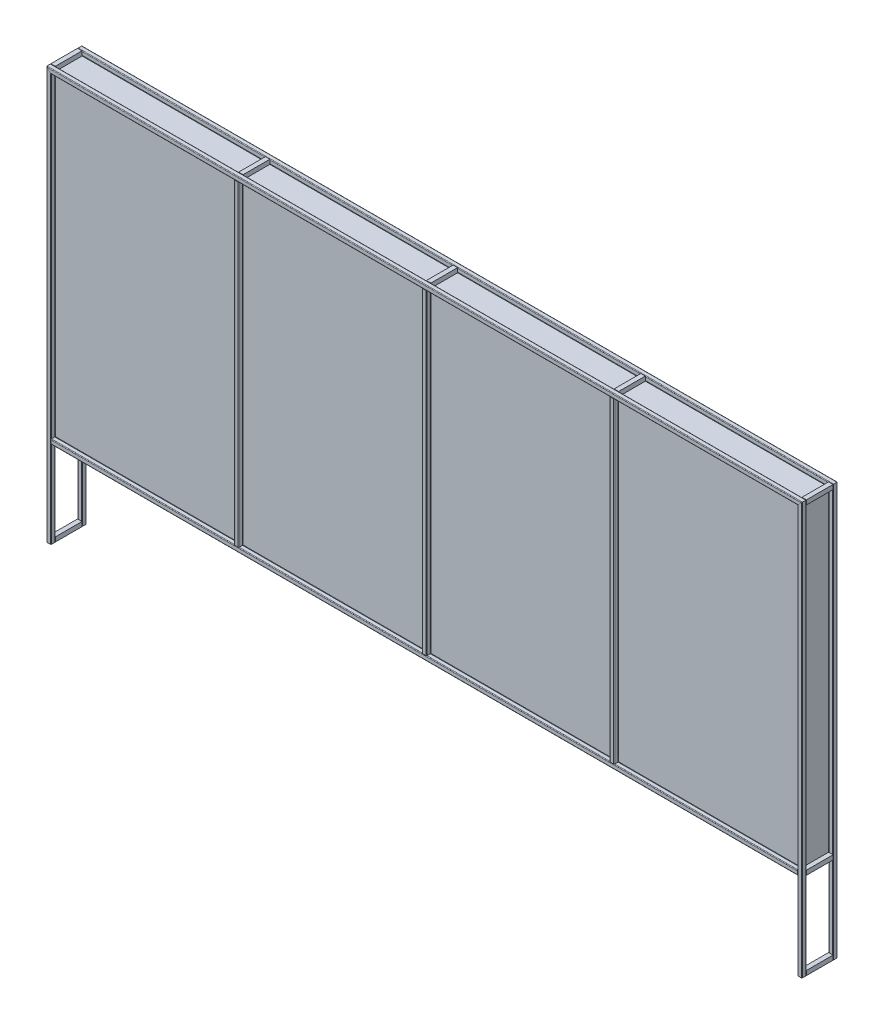
from build123d import *

# Parameters (mm, degrees)
GB_6728_1986_025_X_25_X_1_75_1_DEPTH        = 2318.67766953
GB_6728_1986_025_X_25_X_1_75_1_2_DEPTH      = 4252.355339059
GB_6728_1986_025_X_25_X_1_75_1_3_DEPTH      = 2300
GB_6728_1986_025_X_25_X_1_75_1_3_DEPTH_BACK = 18.67766953
GB_6728_1986_025_X_25_X_1_75_1_4_DEPTH      = 4217
GB_6728_1986_025_X_25_X_1_75_1_5_DEPTH      = 1802
GB_6728_1986_025_X_25_X_1_75_1_6_DEPTH      = 1802
GB_6728_1986_025_X_25_X_1_75_1_7_DEPTH      = 1802
PATTERN_LINEAR_1_COUNT                      = 2
PATTERN_LINEAR_1_PITCH                      = 175
SKETCH_2_W                                  = 25
SKETCH_2_H                                  = 25
EXTRUDE_1_DEPTH                             = 150
EXTRUDE_1_2_DEPTH                           = 150
EXTRUDE_1_3_DEPTH                           = 150
EXTRUDE_1_4_DEPTH                           = 150
EXTRUDE_1_5_DEPTH                           = 150
EXTRUDE_1_6_DEPTH                           = 150
EXTRUDE_1_7_DEPTH                           = 150
EXTRUDE_1_8_DEPTH                           = 150
EXTRUDE_1_9_DEPTH                           = 150
EXTRUDE_1_10_DEPTH                          = 150
EXTRUDE_1_11_DEPTH                          = 150
EXTRUDE_1_12_DEPTH                          = 150
SKETCH_3_W                                  = 1028.75
SKETCH_3_H                                  = 1775
EXTRUDE_2_DEPTH                             = 150
PATTERN_LINEAR_3_COUNT                      = 4
PATTERN_LINEAR_3_PITCH                      = 1053.75


with BuildPart() as part:
    # Sketch1 on segment 1 (carried to segment 1) → Gb／6728-1986方形空心型钢 025 X 25 X 1.75(1) (new body)
    with BuildSketch(Plane(origin=(2107.5, 0, 0), x_dir=(-1, 0, 0), z_dir=(0, 1, 0))):
        with BuildLine():
            Line((-9, -12.5), (9, -12.5))
            ThreePointArc((9, -12.5), (11.474873734, -11.474873734), (12.5, -9))
            Line((12.5, -9), (12.5, 9))
            ThreePointArc((12.5, 9), (11.474873734, 11.474873734), (9, 12.5))
            Line((9, 12.5), (-9, 12.5))
            ThreePointArc((-9, 12.5), (-11.474873734, 11.474873734), (-12.5, 9))
            Line((-12.5, 9), (-12.5, -9))
            ThreePointArc((-12.5, -9), (-11.474873734, -11.474873734), (-9, -12.5))
        make_face()
        with BuildLine():
            Line((-9, -10.75), (9, -10.75))
            ThreePointArc((9, -10.75), (10.237436867, -10.237436867), (10.75, -9))
            Line((10.75, -9), (10.75, 9))
            ThreePointArc((10.75, 9), (10.237436867, 10.237436867), (9, 10.75))
            Line((9, 10.75), (-9, 10.75))
            ThreePointArc((-9, 10.75), (-10.237436867, 10.237436867), (-10.75, 9))
            Line((-10.75, 9), (-10.75, -9))
            ThreePointArc((-10.75, -9), (-10.237436867, -10.237436867), (-9, -10.75))
        make_face(mode=Mode.SUBTRACT)
    extrude(amount=GB_6728_1986_025_X_25_X_1_75_1_DEPTH)

    # Gb／6728-1986方形空心型钢 025 X 25 X 1.75(1) mitre 1
    split(bisect_by=Plane(origin=(2107.5, 2300, 0), x_dir=(0.707106781, 0.707106781, 0), z_dir=(0.707106781, -0.707106781, 0)), keep=Keep.TOP)


with BuildPart() as body_2:
    # Sketch1 on segment 2 (carried to segment 2) → Gb_6728-1986_ 025 X 25 X 1.75_1 2 (new body)
    with BuildSketch(Plane(origin=(2126.17766953, 2300, 0), x_dir=(0, -1, 0), z_dir=(-1, 0, 0))):
        with BuildLine():
            Line((-9, -12.5), (9, -12.5))
            ThreePointArc((9, -12.5), (11.474873734, -11.474873734), (12.5, -9))
            Line((12.5, -9), (12.5, 9))
            ThreePointArc((12.5, 9), (11.474873734, 11.474873734), (9, 12.5))
            Line((9, 12.5), (-9, 12.5))
            ThreePointArc((-9, 12.5), (-11.474873734, 11.474873734), (-12.5, 9))
            Line((-12.5, 9), (-12.5, -9))
            ThreePointArc((-12.5, -9), (-11.474873734, -11.474873734), (-9, -12.5))
        make_face()
        with BuildLine():
            Line((-9, -10.75), (9, -10.75))
            ThreePointArc((9, -10.75), (10.237436867, -10.237436867), (10.75, -9))
            Line((10.75, -9), (10.75, 9))
            ThreePointArc((10.75, 9), (10.237436867, 10.237436867), (9, 10.75))
            Line((9, 10.75), (-9, 10.75))
            ThreePointArc((-9, 10.75), (-10.237436867, 10.237436867), (-10.75, 9))
            Line((-10.75, 9), (-10.75, -9))
            ThreePointArc((-10.75, -9), (-10.237436867, -10.237436867), (-9, -10.75))
        make_face(mode=Mode.SUBTRACT)
    extrude(amount=GB_6728_1986_025_X_25_X_1_75_1_2_DEPTH)

    # Gb_6728-1986_ 025 X 25 X 1.75_1 2 mitre
    split(bisect_by=Plane(origin=(-2107.5, 2300, 0), x_dir=(-0.707106781, 0.707106781, 0), z_dir=(0.707106781, 0.707106781, 0)), keep=Keep.TOP)

    # Gb_6728-1986_ 025 X 25 X 1.75_1 2 mi 2
    split(bisect_by=Plane(origin=(2107.5, 2300, 0), x_dir=(-0.707106781, -0.707106781, 0), z_dir=(-0.707106781, 0.707106781, 0)), keep=Keep.TOP)


with BuildPart() as body_3:
    # Sketch1 → Gb_6728-1986_ 025 X 25 X 1.75_1 3 (new, two sides: drawn at the far end of the back side and taken through both)
    with BuildSketch(Plane(origin=(-2107.5, 2300, 0), x_dir=(1, 0, 0), z_dir=(0, -1, 0)).offset(-GB_6728_1986_025_X_25_X_1_75_1_3_DEPTH_BACK)):
        with BuildLine():
            Line((-9, -12.5), (9, -12.5))
            ThreePointArc((9, -12.5), (11.474873734, -11.474873734), (12.5, -9))
            Line((12.5, -9), (12.5, 9))
            ThreePointArc((12.5, 9), (11.474873734, 11.474873734), (9, 12.5))
            Line((9, 12.5), (-9, 12.5))
            ThreePointArc((-9, 12.5), (-11.474873734, 11.474873734), (-12.5, 9))
            Line((-12.5, 9), (-12.5, -9))
            ThreePointArc((-12.5, -9), (-11.474873734, -11.474873734), (-9, -12.5))
        make_face()
        with BuildLine():
            Line((-9, -10.75), (9, -10.75))
            ThreePointArc((9, -10.75), (10.237436867, -10.237436867), (10.75, -9))
            Line((10.75, -9), (10.75, 9))
            ThreePointArc((10.75, 9), (10.237436867, 10.237436867), (9, 10.75))
            Line((9, 10.75), (-9, 10.75))
            ThreePointArc((-9, 10.75), (-10.237436867, 10.237436867), (-10.75, 9))
            Line((-10.75, 9), (-10.75, -9))
            ThreePointArc((-10.75, -9), (-10.237436867, -10.237436867), (-9, -10.75))
        make_face(mode=Mode.SUBTRACT)
    extrude(amount=GB_6728_1986_025_X_25_X_1_75_1_3_DEPTH + GB_6728_1986_025_X_25_X_1_75_1_3_DEPTH_BACK)

    # Gb_6728-1986_ 025 X 25 X 1.75_1 3 mitre
    split(bisect_by=Plane(origin=(-2107.5, 2300, 0), x_dir=(0.707106781, -0.707106781, 0), z_dir=(-0.707106781, -0.707106781, 0)), keep=Keep.TOP)


with BuildPart() as body_4:
    # Sketch1 on segment 4 (carried to segment 4) → Gb_6728-1986_ 025 X 25 X 1.75_1 4 (new body)
    with BuildSketch(Plane(origin=(-2108.5, 500, 0), x_dir=(0, 1, 0), z_dir=(1, 0, 0))):
        with BuildLine():
            Line((-9, -12.5), (9, -12.5))
            ThreePointArc((9, -12.5), (11.474873734, -11.474873734), (12.5, -9))
            Line((12.5, -9), (12.5, 9))
            ThreePointArc((12.5, 9), (11.474873734, 11.474873734), (9, 12.5))
            Line((9, 12.5), (-9, 12.5))
            ThreePointArc((-9, 12.5), (-11.474873734, 11.474873734), (-12.5, 9))
            Line((-12.5, 9), (-12.5, -9))
            ThreePointArc((-12.5, -9), (-11.474873734, -11.474873734), (-9, -12.5))
        make_face()
        with BuildLine():
            Line((-9, -10.75), (9, -10.75))
            ThreePointArc((9, -10.75), (10.237436867, -10.237436867), (10.75, -9))
            Line((10.75, -9), (10.75, 9))
            ThreePointArc((10.75, 9), (10.237436867, 10.237436867), (9, 10.75))
            Line((9, 10.75), (-9, 10.75))
            ThreePointArc((-9, 10.75), (-10.237436867, 10.237436867), (-10.75, 9))
            Line((-10.75, 9), (-10.75, -9))
            ThreePointArc((-10.75, -9), (-10.237436867, -10.237436867), (-9, -10.75))
        make_face(mode=Mode.SUBTRACT)
    extrude(amount=GB_6728_1986_025_X_25_X_1_75_1_4_DEPTH)

    # Gb_6728-1986_ 025 X 25 X 1.75_1 4 mitre
    split(bisect_by=Plane(origin=(-2095, 500, 0), x_dir=(0, 1, 0), z_dir=(1, 0, 0)), keep=Keep.TOP)

    # Gb_6728-1986_ 025 X 25 X 1.75_1 4 mi 2
    split(bisect_by=Plane(origin=(2095, 500, 0), x_dir=(0, -1, 0), z_dir=(-1, 0, 0)), keep=Keep.TOP)


with BuildPart() as body_5:
    # Sketch1 on segment 5 (carried to segment 5) → Gb_6728-1986_ 025 X 25 X 1.75_1 5 (new body)
    with BuildSketch(Plane(origin=(-1053.75, 2301, 0), x_dir=(1, 0, 0), z_dir=(0, -1, 0))):
        with BuildLine():
            Line((-9, -12.5), (9, -12.5))
            ThreePointArc((9, -12.5), (11.474873734, -11.474873734), (12.5, -9))
            Line((12.5, -9), (12.5, 9))
            ThreePointArc((12.5, 9), (11.474873734, 11.474873734), (9, 12.5))
            Line((9, 12.5), (-9, 12.5))
            ThreePointArc((-9, 12.5), (-11.474873734, 11.474873734), (-12.5, 9))
            Line((-12.5, 9), (-12.5, -9))
            ThreePointArc((-12.5, -9), (-11.474873734, -11.474873734), (-9, -12.5))
        make_face()
        with BuildLine():
            Line((-9, -10.75), (9, -10.75))
            ThreePointArc((9, -10.75), (10.237436867, -10.237436867), (10.75, -9))
            Line((10.75, -9), (10.75, 9))
            ThreePointArc((10.75, 9), (10.237436867, 10.237436867), (9, 10.75))
            Line((9, 10.75), (-9, 10.75))
            ThreePointArc((-9, 10.75), (-10.237436867, 10.237436867), (-10.75, 9))
            Line((-10.75, 9), (-10.75, -9))
            ThreePointArc((-10.75, -9), (-10.237436867, -10.237436867), (-9, -10.75))
        make_face(mode=Mode.SUBTRACT)
    extrude(amount=GB_6728_1986_025_X_25_X_1_75_1_5_DEPTH)

    # Gb_6728-1986_ 025 X 25 X 1.75_1 5 mitre
    split(bisect_by=Plane(origin=(-1053.75, 2287.5, 0), x_dir=(1, 0, 0), z_dir=(0, -1, 0)), keep=Keep.TOP)

    # Gb_6728-1986_ 025 X 25 X 1.75_1 5 mi 2
    split(bisect_by=Plane(origin=(-1053.75, 512.5, 0), x_dir=(-1, 0, 0), z_dir=(0, 1, 0)), keep=Keep.TOP)


with BuildPart() as body_6:
    # Sketch1 on segment 6 (carried to segment 6) → Gb_6728-1986_ 025 X 25 X 1.75_1 6 (new body)
    with BuildSketch(Plane(origin=(0, 499, 0), x_dir=(-1, 0, 0), z_dir=(0, 1, 0))):
        with BuildLine():
            Line((-9, -12.5), (9, -12.5))
            ThreePointArc((9, -12.5), (11.474873734, -11.474873734), (12.5, -9))
            Line((12.5, -9), (12.5, 9))
            ThreePointArc((12.5, 9), (11.474873734, 11.474873734), (9, 12.5))
            Line((9, 12.5), (-9, 12.5))
            ThreePointArc((-9, 12.5), (-11.474873734, 11.474873734), (-12.5, 9))
            Line((-12.5, 9), (-12.5, -9))
            ThreePointArc((-12.5, -9), (-11.474873734, -11.474873734), (-9, -12.5))
        make_face()
        with BuildLine():
            Line((-9, -10.75), (9, -10.75))
            ThreePointArc((9, -10.75), (10.237436867, -10.237436867), (10.75, -9))
            Line((10.75, -9), (10.75, 9))
            ThreePointArc((10.75, 9), (10.237436867, 10.237436867), (9, 10.75))
            Line((9, 10.75), (-9, 10.75))
            ThreePointArc((-9, 10.75), (-10.237436867, 10.237436867), (-10.75, 9))
            Line((-10.75, 9), (-10.75, -9))
            ThreePointArc((-10.75, -9), (-10.237436867, -10.237436867), (-9, -10.75))
        make_face(mode=Mode.SUBTRACT)
    extrude(amount=GB_6728_1986_025_X_25_X_1_75_1_6_DEPTH)

    # Gb_6728-1986_ 025 X 25 X 1.75_1 6 mitre
    split(bisect_by=Plane(origin=(0, 512.5, 0), x_dir=(-1, 0, 0), z_dir=(0, 1, 0)), keep=Keep.TOP)

    # Gb_6728-1986_ 025 X 25 X 1.75_1 6 mi 2
    split(bisect_by=Plane.XZ.offset(-2287.5), keep=Keep.TOP)


with BuildPart() as body_7:
    # Sketch1 on segment 7 (carried to segment 7) → Gb_6728-1986_ 025 X 25 X 1.75_1 7 (new body)
    with BuildSketch(Plane(origin=(1053.75, 2301, 0), x_dir=(1, 0, 0), z_dir=(0, -1, 0))):
        with BuildLine():
            Line((-9, -12.5), (9, -12.5))
            ThreePointArc((9, -12.5), (11.474873734, -11.474873734), (12.5, -9))
            Line((12.5, -9), (12.5, 9))
            ThreePointArc((12.5, 9), (11.474873734, 11.474873734), (9, 12.5))
            Line((9, 12.5), (-9, 12.5))
            ThreePointArc((-9, 12.5), (-11.474873734, 11.474873734), (-12.5, 9))
            Line((-12.5, 9), (-12.5, -9))
            ThreePointArc((-12.5, -9), (-11.474873734, -11.474873734), (-9, -12.5))
        make_face()
        with BuildLine():
            Line((-9, -10.75), (9, -10.75))
            ThreePointArc((9, -10.75), (10.237436867, -10.237436867), (10.75, -9))
            Line((10.75, -9), (10.75, 9))
            ThreePointArc((10.75, 9), (10.237436867, 10.237436867), (9, 10.75))
            Line((9, 10.75), (-9, 10.75))
            ThreePointArc((-9, 10.75), (-10.237436867, 10.237436867), (-10.75, 9))
            Line((-10.75, 9), (-10.75, -9))
            ThreePointArc((-10.75, -9), (-10.237436867, -10.237436867), (-9, -10.75))
        make_face(mode=Mode.SUBTRACT)
    extrude(amount=GB_6728_1986_025_X_25_X_1_75_1_7_DEPTH)

    # Gb_6728-1986_ 025 X 25 X 1.75_1 7 mitre
    split(bisect_by=Plane(origin=(1053.75, 2287.5, 0), x_dir=(1, 0, 0), z_dir=(0, -1, 0)), keep=Keep.TOP)

    # Gb_6728-1986_ 025 X 25 X 1.75_1 7 mi 2
    split(bisect_by=Plane(origin=(1053.75, 512.5, 0), x_dir=(-1, 0, 0), z_dir=(0, 1, 0)), keep=Keep.TOP)


with BuildPart() as pattern_linear_1_1:
    # 阵列(线性)1: pattern copy
    add(body_5.part.moved(Location(Vector(0, 0, -1) * (1 * PATTERN_LINEAR_1_PITCH))))


with BuildPart() as pattern_linear_1_2:
    # 阵列(线性)1: pattern copy
    add(body_7.part.moved(Location(Vector(0, 0, -1) * (1 * PATTERN_LINEAR_1_PITCH))))


with BuildPart() as pattern_linear_1_3:
    # 阵列(线性)1: pattern copy
    add(body_6.part.moved(Location(Vector(0, 0, -1) * (1 * PATTERN_LINEAR_1_PITCH))))


with BuildPart() as pattern_linear_1_4:
    # 阵列(线性)1: pattern copy
    add(part.part.moved(Location(Vector(0, 0, -1) * (1 * PATTERN_LINEAR_1_PITCH))))


with BuildPart() as pattern_linear_1_5:
    # 阵列(线性)1: pattern copy
    add(body_4.part.moved(Location(Vector(0, 0, -1) * (1 * PATTERN_LINEAR_1_PITCH))))


with BuildPart() as pattern_linear_1_6:
    # 阵列(线性)1: pattern copy
    add(body_3.part.moved(Location(Vector(0, 0, -1) * (1 * PATTERN_LINEAR_1_PITCH))))


with BuildPart() as pattern_linear_1_7:
    # 阵列(线性)1: pattern copy
    add(body_2.part.moved(Location(Vector(0, 0, -1) * (1 * PATTERN_LINEAR_1_PITCH))))


with BuildPart() as body_15:
    # 草图2 → 凸台-拉伸1 (new body)
    with BuildSketch(Plane.XY.offset(-162.5)):
        with Locations((-2107.5, 2300)):
            Rectangle(SKETCH_2_W, SKETCH_2_H)
    extrude(amount=EXTRUDE_1_DEPTH)


with BuildPart() as body_16:
    # 草图2 → Extrude 1 2 (new body)
    with BuildSketch(Plane.XY.offset(-162.5)):
        with Locations((-2107.5, 500)):
            Rectangle(SKETCH_2_W, SKETCH_2_H)
    extrude(amount=EXTRUDE_1_2_DEPTH)


with BuildPart() as body_17:
    # 草图2 → Extrude 1 3 (new body)
    with BuildSketch(Plane.XY.offset(-162.5)):
        with Locations((-2107.5, 12.5)):
            Rectangle(SKETCH_2_W, SKETCH_2_H)
    extrude(amount=EXTRUDE_1_3_DEPTH)


with BuildPart() as body_18:
    # 草图2 → Extrude 1 4 (new body)
    with BuildSketch(Plane.XY.offset(-162.5)):
        with Locations((2107.5, 12.5)):
            Rectangle(SKETCH_2_W, SKETCH_2_H)
    extrude(amount=EXTRUDE_1_4_DEPTH)


with BuildPart() as body_19:
    # 草图2 → Extrude 1 5 (new body)
    with BuildSketch(Plane.XY.offset(-162.5)):
        with Locations((2107.5, 500)):
            Rectangle(SKETCH_2_W, SKETCH_2_H)
    extrude(amount=EXTRUDE_1_5_DEPTH)


with BuildPart() as body_20:
    # 草图2 → Extrude 1 6 (new body)
    with BuildSketch(Plane.XY.offset(-162.5)):
        with Locations((2107.5, 2300)):
            Rectangle(SKETCH_2_W, SKETCH_2_H)
    extrude(amount=EXTRUDE_1_6_DEPTH)


with BuildPart() as body_21:
    # 草图2 → Extrude 1 7 (new body)
    with BuildSketch(Plane.XY.offset(-162.5)):
        with Locations((-1053.75, 2300)):
            Rectangle(SKETCH_2_W, SKETCH_2_H)
    extrude(amount=EXTRUDE_1_7_DEPTH)


with BuildPart() as body_22:
    # 草图2 → Extrude 1 8 (new body)
    with BuildSketch(Plane.XY.offset(-162.5)):
        with Locations((-1053.75, 500)):
            Rectangle(SKETCH_2_W, SKETCH_2_H)
    extrude(amount=EXTRUDE_1_8_DEPTH)


with BuildPart() as body_23:
    # 草图2 → Extrude 1 9 (new body)
    with BuildSketch(Plane.XY.offset(-162.5)):
        with Locations((1053.75, 500)):
            Rectangle(SKETCH_2_W, SKETCH_2_H)
    extrude(amount=EXTRUDE_1_9_DEPTH)


with BuildPart() as body_24:
    # 草图2 → Extrude 1 10 (new body)
    with BuildSketch(Plane.XY.offset(-162.5)):
        with Locations((1053.75, 2300)):
            Rectangle(SKETCH_2_W, SKETCH_2_H)
    extrude(amount=EXTRUDE_1_10_DEPTH)


with BuildPart() as body_25:
    # 草图2 → Extrude 1 11 (new body)
    with BuildSketch(Plane.XY.offset(-162.5)):
        with Locations((0, 500)):
            Rectangle(SKETCH_2_W, SKETCH_2_H)
    extrude(amount=EXTRUDE_1_11_DEPTH)


with BuildPart() as body_26:
    # 草图2 → Extrude 1 12 (new body)
    with BuildSketch(Plane.XY.offset(-162.5)):
        with Locations((0, 2300)):
            Rectangle(SKETCH_2_W, SKETCH_2_H)
    extrude(amount=EXTRUDE_1_12_DEPTH)


with BuildPart() as body_27:
    # 草图3 → 凸台-拉伸2 (new body)
    with BuildSketch(Plane(origin=(0, 0, -12.5), x_dir=(-1, 0, 0), z_dir=(0, 0, -1))):
        with Locations((-1580.625, 1400)):
            Rectangle(SKETCH_3_W, SKETCH_3_H)
    extrude(amount=EXTRUDE_2_DEPTH)


with BuildPart() as pattern_linear_3_1:
    # 阵列(线性)3: pattern copy
    add(body_27.part.moved(Location(Vector(-1, 0, 0) * (1 * PATTERN_LINEAR_3_PITCH))))


with BuildPart() as pattern_linear_3_2:
    # 阵列(线性)3: pattern copy
    add(body_27.part.moved(Location(Vector(-1, 0, 0) * (2 * PATTERN_LINEAR_3_PITCH))))


with BuildPart() as pattern_linear_3_3:
    # 阵列(线性)3: pattern copy
    add(body_27.part.moved(Location(Vector(-1, 0, 0) * (3 * PATTERN_LINEAR_3_PITCH))))


solid = Compound([part.part, body_2.part, body_3.part, body_4.part, body_5.part, body_6.part, body_7.part, pattern_linear_1_1.part, pattern_linear_1_2.part, pattern_linear_1_3.part, pattern_linear_1_4.part, pattern_linear_1_5.part, pattern_linear_1_6.part, pattern_linear_1_7.part, body_15.part, body_16.part, body_17.part, body_18.part, body_19.part, body_20.part, body_21.part, body_22.part, body_23.part, body_24.part, body_25.part, body_26.part, body_27.part, pattern_linear_3_1.part, pattern_linear_3_2.part, pattern_linear_3_3.part])
